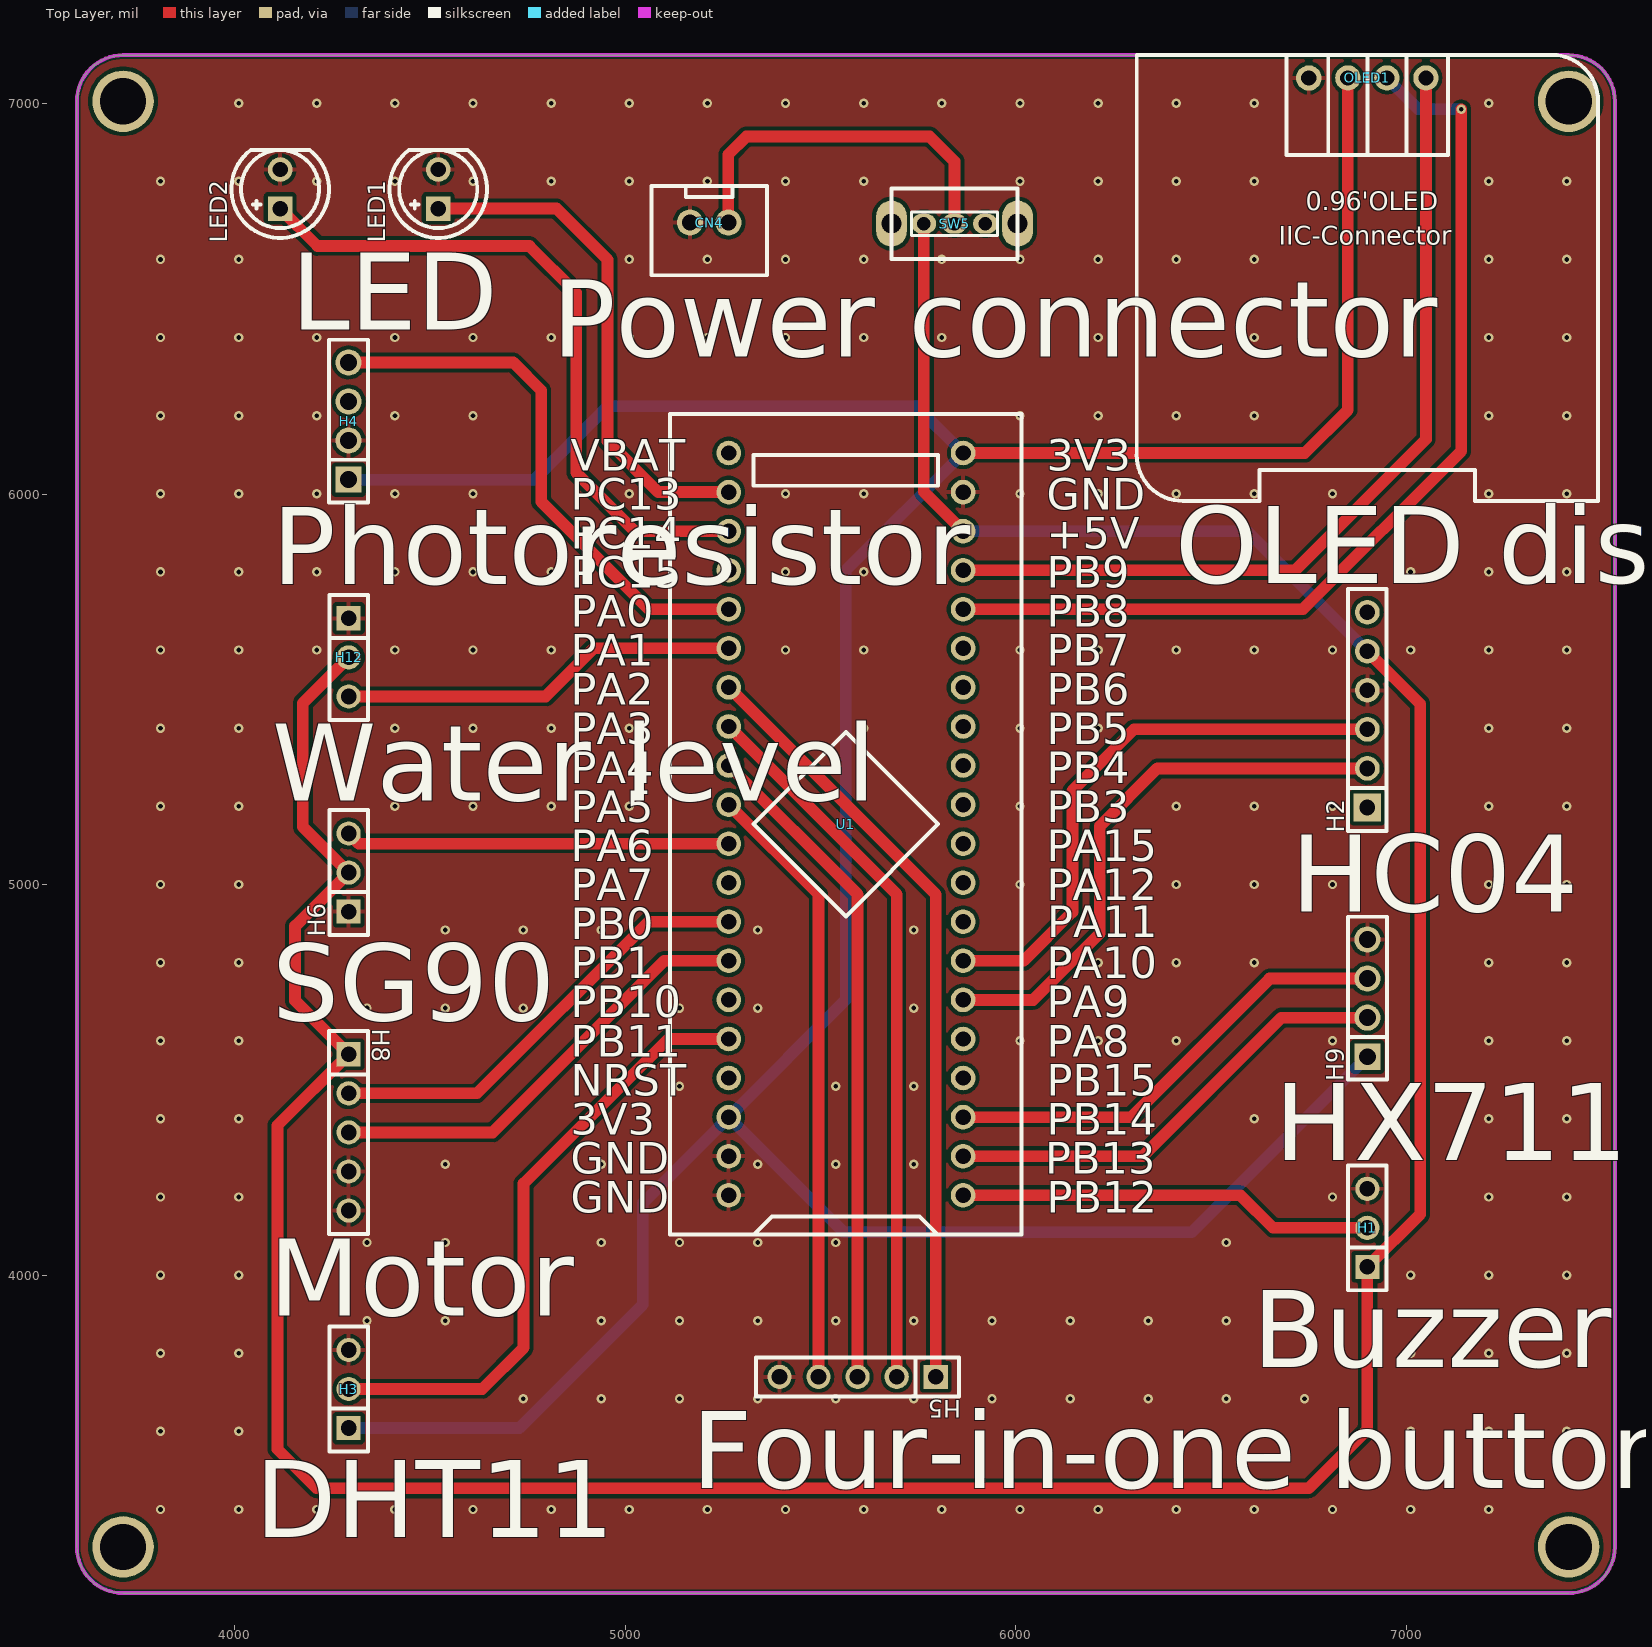
[diagram p0: Top Layer view]
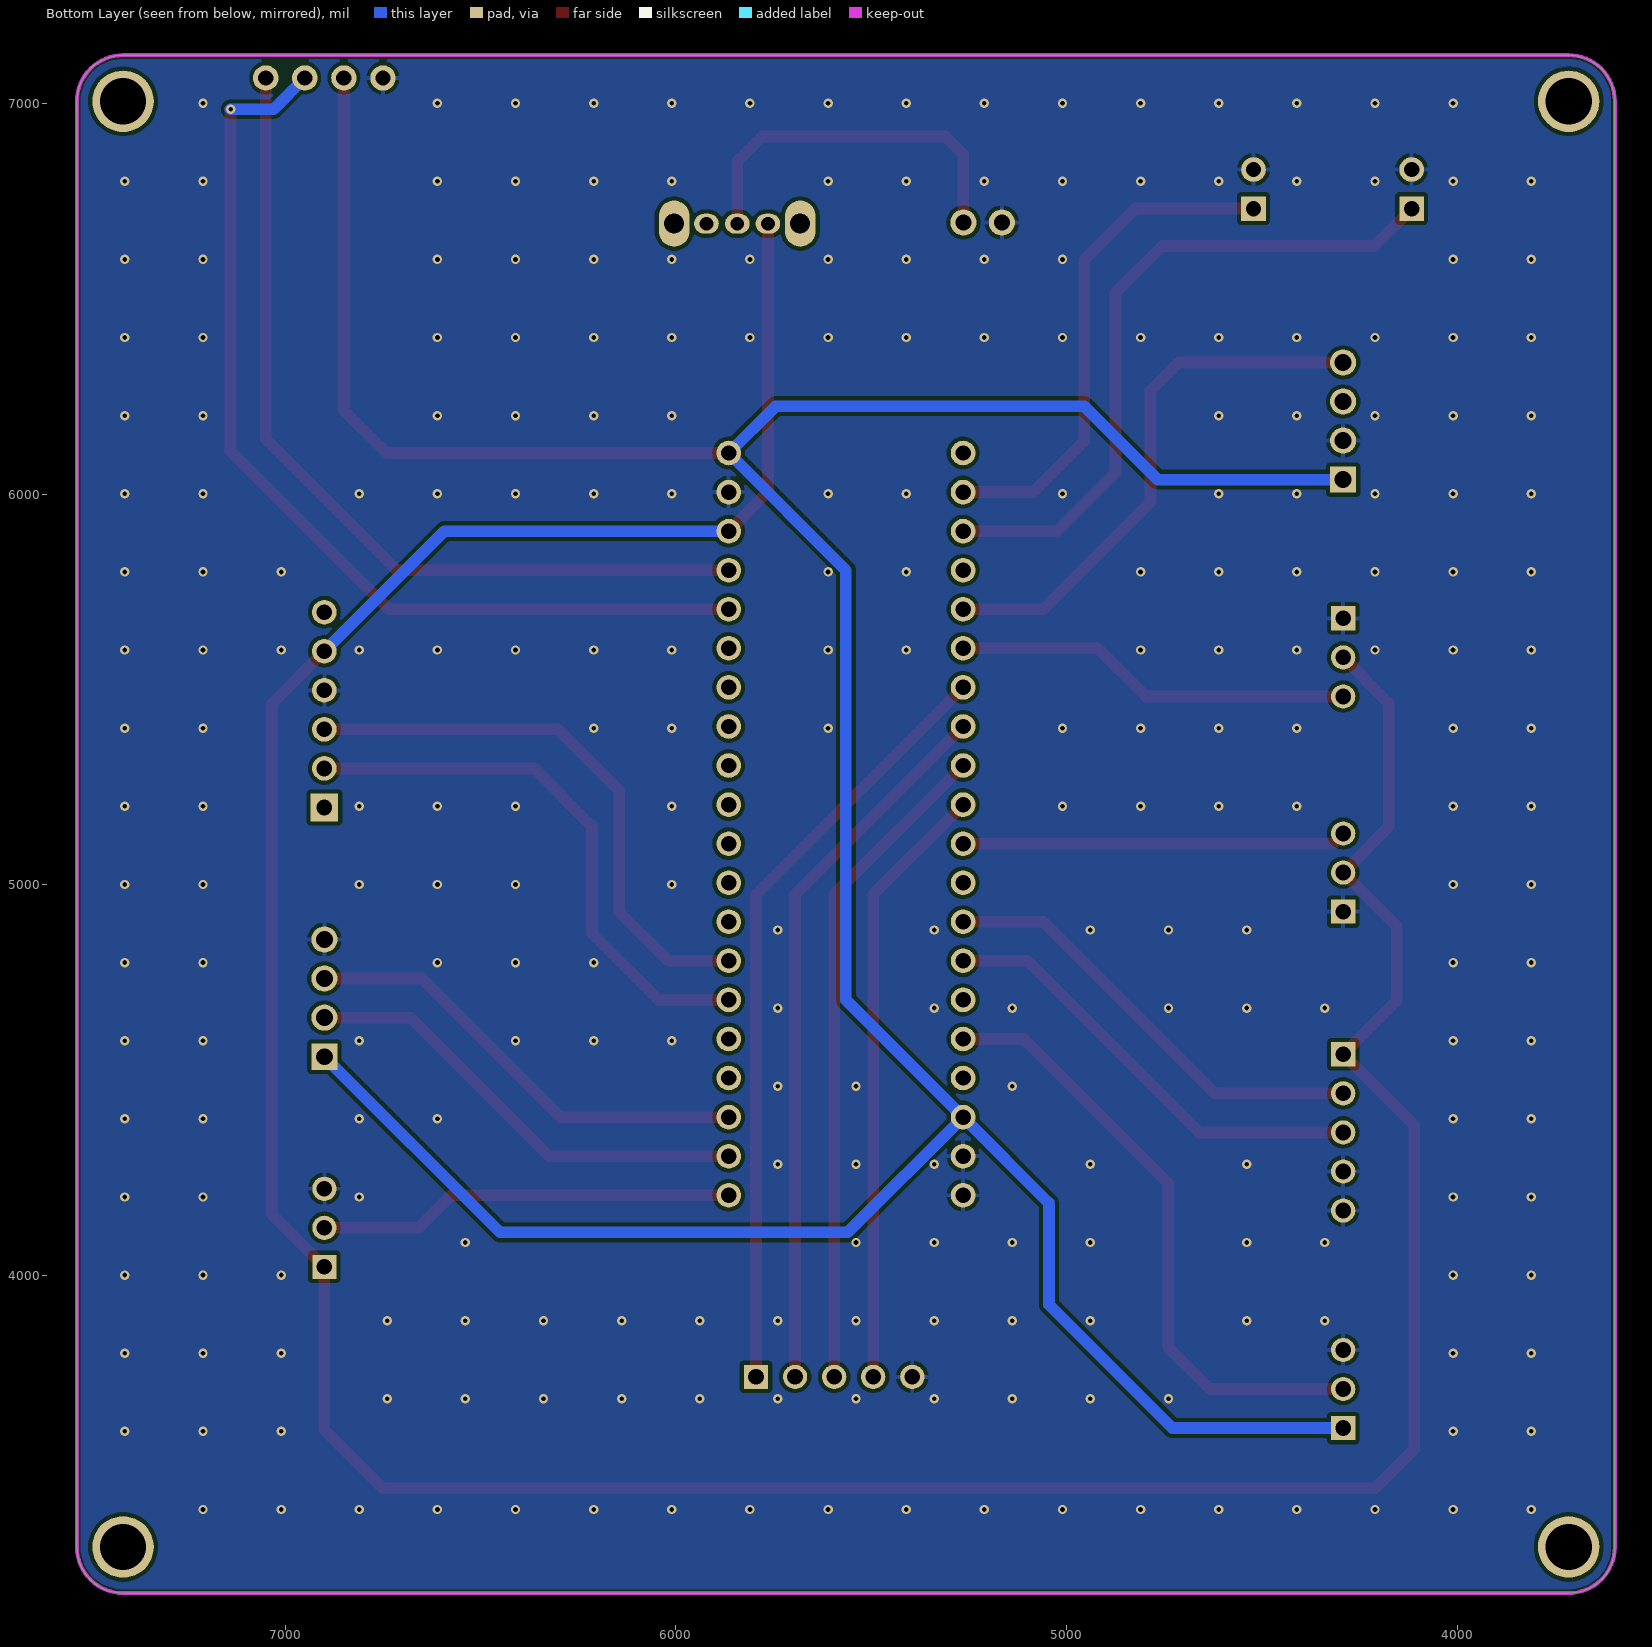
[diagram p1: Bottom Layer view, seen from below]
# Altium PCB MISC51952.pcbdoc
Units mil, origin at the board's own origin, x right, y up, seen from the top; angles counter-clockwise.
Board outline 3937.01 x 3937.01 mil, 2 copper layers (Top Layer, Bottom Layer), stack 62.206 mil thick; 15 components, 38 nets, 95 pads, 254 vias.

## Layer stack, top to bottom
Top Solder Mask Layer: solder mask 0.394, Dk 3.3
Top Layer: signal copper 1.379
Dielectric1: surface 59.449, FR4, Dk 4.5
Bottom Layer: signal copper 1.378
Bottom Solder Mask Layer: solder mask 0.394, Dk 3.3

## Board outline
3714.61,7123.5 ccw(c3714.61,7005.39) 3596.5,7005.39 3596.5,3304.61 ccw(c3714.61,3304.61) 3714.61,3186.5 7415.39,3186.5 ccw(c7415.39,3304.61) 7533.5,3304.61 7533.5,7005.39 ccw(c7415.39,7005.39) 7415.39,7123.5 3714.61,7123.5

## Design rules (kind name [scope] priority, off if disabled: settings)
BoardOutlineClearance copperThickness2oz_1 [All] p2 off: genericclearance=7.99 ignorepadtopadclearanceinfootprint=FALSE except(0: Arc-SplitContinuation Track-SplitContinuation SMDPad-SplitContinuation THPad-SplitContinuation Via-SplitContinuation Fill-SplitContinuation Region-SplitContinuation Poly-SplitContinuation Text-SplitContinuation Hole-SplitContinuation; 5.98: Arc-CutoutEdge Track-CutoutEdge SMDPad-CutoutEdge THPad-CutoutEdge Via-CutoutEdge Text-CutoutEdge; 6.9: Hole-OutlineEdge Hole-CutoutEdge; 10: Poly-OutlineEdge Poly-CutoutEdge; 11.81: Arc-OutlineEdge Track-OutlineEdge SMDPad-OutlineEdge THPad-OutlineEdge Via-OutlineEdge Fill-OutlineEdge Region-OutlineEdge Text-OutlineEdge Fill-CutoutEdge Region-CutoutEdge)
BoardOutlineClearance Plane_innerPlane_1 [All] p4 off: genericclearance=4.02 ignorepadtopadclearanceinfootprint=FALSE except(0: Arc-SplitContinuation Track-SplitContinuation SMDPad-SplitContinuation THPad-SplitContinuation Via-SplitContinuation Fill-SplitContinuation Region-SplitContinuation Poly-SplitContinuation Text-SplitContinuation Hole-SplitContinuation; 5.98: Arc-CutoutEdge Track-CutoutEdge SMDPad-CutoutEdge THPad-CutoutEdge Via-CutoutEdge Text-CutoutEdge; 6.9: Hole-OutlineEdge Hole-CutoutEdge; 10: Poly-OutlineEdge Poly-CutoutEdge; 11.81: Arc-OutlineEdge Track-OutlineEdge SMDPad-OutlineEdge THPad-OutlineEdge Via-OutlineEdge Fill-OutlineEdge Region-OutlineEdge Text-OutlineEdge Fill-CutoutEdge Region-CutoutEdge)
BoardOutlineClearance Copper_copperRegion_1 [All] p6 off: genericclearance=4.02 ignorepadtopadclearanceinfootprint=FALSE except(0: Arc-SplitContinuation Track-SplitContinuation SMDPad-SplitContinuation THPad-SplitContinuation Via-SplitContinuation Fill-SplitContinuation Region-SplitContinuation Poly-SplitContinuation Text-SplitContinuation Hole-SplitContinuation; 5.98: Arc-CutoutEdge Track-CutoutEdge SMDPad-CutoutEdge THPad-CutoutEdge Via-CutoutEdge Text-CutoutEdge; 6.9: Hole-OutlineEdge Hole-CutoutEdge; 10: Poly-OutlineEdge Poly-CutoutEdge; 11.81: Arc-OutlineEdge Track-OutlineEdge SMDPad-OutlineEdge THPad-OutlineEdge Via-OutlineEdge Fill-OutlineEdge Region-OutlineEdge Text-OutlineEdge Fill-CutoutEdge Region-CutoutEdge)
BoardOutlineClearance Copper_copperRegion_copperThickness1oz_1 [All] p8 off: genericclearance=4.02 ignorepadtopadclearanceinfootprint=FALSE except(0: Arc-SplitContinuation Track-SplitContinuation SMDPad-SplitContinuation THPad-SplitContinuation Via-SplitContinuation Fill-SplitContinuation Region-SplitContinuation Poly-SplitContinuation Text-SplitContinuation Hole-SplitContinuation; 5.98: Arc-CutoutEdge Track-CutoutEdge SMDPad-CutoutEdge THPad-CutoutEdge Via-CutoutEdge Text-CutoutEdge; 6.9: Hole-OutlineEdge Hole-CutoutEdge; 10: Poly-OutlineEdge Poly-CutoutEdge; 11.81: Arc-OutlineEdge Track-OutlineEdge SMDPad-OutlineEdge THPad-OutlineEdge Via-OutlineEdge Fill-OutlineEdge Region-OutlineEdge Text-OutlineEdge Fill-CutoutEdge Region-CutoutEdge)
BoardOutlineClearance Copper_copperRegion_Copper_copperRegion_1 [All] p10 off: genericclearance=4.02 ignorepadtopadclearanceinfootprint=FALSE except(0: Arc-SplitContinuation Track-SplitContinuation SMDPad-SplitContinuation THPad-SplitContinuation Via-SplitContinuation Fill-SplitContinuation Region-SplitContinuation Poly-SplitContinuation Text-SplitContinuation Hole-SplitContinuation; 5.98: Arc-CutoutEdge Track-CutoutEdge SMDPad-CutoutEdge THPad-CutoutEdge Via-CutoutEdge Text-CutoutEdge; 6.9: Hole-OutlineEdge Hole-CutoutEdge; 10: Poly-OutlineEdge Poly-CutoutEdge; 11.81: Arc-OutlineEdge Track-OutlineEdge SMDPad-OutlineEdge THPad-OutlineEdge Via-OutlineEdge Fill-OutlineEdge Region-OutlineEdge Text-OutlineEdge Fill-CutoutEdge Region-CutoutEdge)
BoardOutlineClearance copperThickness1oz_1 [All] p12: genericclearance=4.02 ignorepadtopadclearanceinfootprint=FALSE except(0: Arc-SplitContinuation Track-SplitContinuation SMDPad-SplitContinuation THPad-SplitContinuation Via-SplitContinuation Fill-SplitContinuation Region-SplitContinuation Poly-SplitContinuation Text-SplitContinuation Hole-SplitContinuation; 5.98: Arc-CutoutEdge Track-CutoutEdge SMDPad-CutoutEdge THPad-CutoutEdge Via-CutoutEdge Text-CutoutEdge; 6.9: Hole-OutlineEdge Hole-CutoutEdge; 10: Poly-OutlineEdge Poly-CutoutEdge; 11.81: Arc-OutlineEdge Track-OutlineEdge SMDPad-OutlineEdge THPad-OutlineEdge Via-OutlineEdge Fill-OutlineEdge Region-OutlineEdge Text-OutlineEdge Fill-CutoutEdge Region-CutoutEdge)
Clearance copperThickness2oz [All] p1 off: gap=7.99 ignorepadtopadclearanceinfootprint=FALSE except(5.98: SMDPad-Track SMDPad-SMDPad THPad-Track SMDPad-THPad THPad-THPad Track-Via SMDPad-Via THPad-Via Via-Via Fill-SMDPad Region-SMDPad Fill-THPad Region-THPad Fill-Via Region-Via Fill-Fill Fill-Region Region-Region Arc-Track Arc-SMDPad Arc-THPad Arc-Via Fill-Arc Region-Arc Arc-Arc Text-Track SMDPad-Text Text-THPad Text-Via Fill-Text Region-Text Arc-Text Text-Text; 6.9: Hole-Track Hole-SMDPad Hole-THPad Hole-Via Fill-Hole Region-Hole Hole-Arc Hole-Text; 10: Poly-Track Poly-SMDPad Poly-THPad Poly-Via Poly-Fill Poly-Region Poly-Poly Poly-Arc Poly-Text Poly-Hole; 11.81: Fill-Track Region-Track)
Clearance Plane_innerPlane [All] p3 off: gap=4.02 ignorepadtopadclearanceinfootprint=FALSE except(5.98: SMDPad-Track SMDPad-SMDPad THPad-Track SMDPad-THPad THPad-THPad Track-Via SMDPad-Via THPad-Via Via-Via Fill-SMDPad Region-SMDPad Fill-THPad Region-THPad Fill-Via Region-Via Fill-Fill Fill-Region Region-Region Arc-Track Arc-SMDPad Arc-THPad Arc-Via Fill-Arc Region-Arc Arc-Arc Text-Track SMDPad-Text Text-THPad Text-Via Fill-Text Region-Text Arc-Text Text-Text; 6.9: Hole-Track Hole-SMDPad Hole-THPad Hole-Via Fill-Hole Region-Hole Hole-Arc Hole-Text; 10: Poly-Track Poly-SMDPad Poly-THPad Poly-Via Poly-Fill Poly-Region Poly-Poly Poly-Arc Poly-Text Poly-Hole; 11.81: Fill-Track Region-Track)
Clearance Copper_copperRegion [All] p5 off: gap=4.02 ignorepadtopadclearanceinfootprint=FALSE except(5.98: SMDPad-Track SMDPad-SMDPad THPad-Track SMDPad-THPad THPad-THPad Track-Via SMDPad-Via THPad-Via Via-Via Fill-SMDPad Region-SMDPad Fill-THPad Region-THPad Fill-Via Region-Via Fill-Fill Fill-Region Region-Region Arc-Track Arc-SMDPad Arc-THPad Arc-Via Fill-Arc Region-Arc Arc-Arc Text-Track SMDPad-Text Text-THPad Text-Via Fill-Text Region-Text Arc-Text Text-Text; 6.9: Hole-Track Hole-SMDPad Hole-THPad Hole-Via Fill-Hole Region-Hole Hole-Arc Hole-Text; 10: Poly-Track Poly-SMDPad Poly-THPad Poly-Via Poly-Fill Poly-Region Poly-Poly Poly-Arc Poly-Text Poly-Hole; 11.81: Fill-Track Region-Track)
Clearance Copper_copperRegion_copperThickness1oz [All] p7 off: gap=4.02 ignorepadtopadclearanceinfootprint=FALSE except(5.98: SMDPad-Track SMDPad-SMDPad THPad-Track SMDPad-THPad THPad-THPad Track-Via SMDPad-Via THPad-Via Via-Via Fill-SMDPad Region-SMDPad Fill-THPad Region-THPad Fill-Via Region-Via Fill-Fill Fill-Region Region-Region Arc-Track Arc-SMDPad Arc-THPad Arc-Via Fill-Arc Region-Arc Arc-Arc Text-Track SMDPad-Text Text-THPad Text-Via Fill-Text Region-Text Arc-Text Text-Text; 6.9: Hole-Track Hole-SMDPad Hole-THPad Hole-Via Fill-Hole Region-Hole Hole-Arc Hole-Text; 10: Poly-Track Poly-SMDPad Poly-THPad Poly-Via Poly-Fill Poly-Region Poly-Poly Poly-Arc Poly-Text Poly-Hole; 11.81: Fill-Track Region-Track)
Clearance Copper_copperRegion_Copper_copperRegion [All] p9 off: gap=4.02 ignorepadtopadclearanceinfootprint=FALSE except(5.98: SMDPad-Track SMDPad-SMDPad THPad-Track SMDPad-THPad THPad-THPad Track-Via SMDPad-Via THPad-Via Via-Via Fill-SMDPad Region-SMDPad Fill-THPad Region-THPad Fill-Via Region-Via Fill-Fill Fill-Region Region-Region Arc-Track Arc-SMDPad Arc-THPad Arc-Via Fill-Arc Region-Arc Arc-Arc Text-Track SMDPad-Text Text-THPad Text-Via Fill-Text Region-Text Arc-Text Text-Text; 6.9: Hole-Track Hole-SMDPad Hole-THPad Hole-Via Fill-Hole Region-Hole Hole-Arc Hole-Text; 10: Poly-Track Poly-SMDPad Poly-THPad Poly-Via Poly-Fill Poly-Region Poly-Poly Poly-Arc Poly-Text Poly-Hole; 11.81: Fill-Track Region-Track)
Clearance copperThickness1oz [All] p11: gap=4.02 ignorepadtopadclearanceinfootprint=FALSE except(5.98: SMDPad-Track SMDPad-SMDPad THPad-Track SMDPad-THPad THPad-THPad Track-Via SMDPad-Via THPad-Via Via-Via Fill-SMDPad Region-SMDPad Fill-THPad Region-THPad Fill-Via Region-Via Fill-Fill Fill-Region Region-Region Arc-Track Arc-SMDPad Arc-THPad Arc-Via Fill-Arc Region-Arc Arc-Arc Text-Track SMDPad-Text Text-THPad Text-Via Fill-Text Region-Text Arc-Text Text-Text; 6.9: Hole-Track Hole-SMDPad Hole-THPad Hole-Via Fill-Hole Region-Hole Hole-Arc Hole-Text; 10: Poly-Track Poly-SMDPad Poly-THPad Poly-Via Poly-Fill Poly-Region Poly-Poly Poly-Arc Poly-Text Poly-Hole; 11.81: Fill-Track Region-Track)
DiffPairsRouting differentialPair [All] p1: maxlimit=6 minlimit=6 mostfreqgap=6 toplayer_minwidth=5 toplayer_prefwidth=10 toplayer_maxwidth=100 toplayer_mingap=6 toplayer_prefgap=6 toplayer_maxgap=6 bottomlayer_minwidth=5 bottomlayer_prefwidth=10 bottomlayer_maxwidth=100 bottomlayer_mingap=6 bottomlayer_prefgap=6 bottomlayer_maxgap=6 maxuncoupledlength=10
HoleToHoleClearance otherClearance [All] p1: gap=11.81 allowstackedmicrovias=TRUE
Length netLength [All] p1: minlimit=0 maxlimit=0
PasteMaskExpansion pasteMaskExpansion [All] p1: expansion=0
PlaneConnect innerPlane [All] p1: planeconnectstyle=Relief reliefexpansion=20 reliefentries=4 reliefconductorwidth=10 reliefairgap=10
PolygonConnect copperRegion_copperThickness1oz [All] p1 off: connectstyle=Relief reliefconductorwidth=10 reliefentries=4 polygonreliefangle="90 Angle" airgapwidth=10 via.connectstyle=Relief via.reliefconductorwidth=10 via.reliefentries=4 via.polygonreliefangle="90 Angle" via.airgapwidth=10
PolygonConnect copperRegion_Copper_copperRegion [All] p2 off: connectstyle=Relief reliefconductorwidth=10 reliefentries=4 polygonreliefangle="90 Angle" airgapwidth=10 via.connectstyle=Relief via.reliefconductorwidth=10 via.reliefentries=4 via.polygonreliefangle="90 Angle" via.airgapwidth=10
PolygonConnect copperRegion [All] p3: connectstyle=Relief reliefconductorwidth=10 reliefentries=4 polygonreliefangle="90 Angle" airgapwidth=10 via.connectstyle=Relief via.reliefconductorwidth=10 via.reliefentries=4 via.polygonreliefangle="90 Angle" via.airgapwidth=10
RoutingVias viaSize [All] p1: holewidth=12.01 width=24.02 viastyle="Through Hole" minholewidth=11.81 minwidth=19.68 maxholewidth=248.03 maxwidth=393.7
SolderMaskExpansion solderMaskExpansion [IsVia] p1: expansion=-1000 istentingtop=TRUE
SolderMaskExpansion solderMaskExpansion [All] p2: expansion=2 istentingtop=FALSE
Width copperThickness2oz_2 [All] p1 off: maxlimit=100 minlimit=8 preferedwidth=10
Width copperThickness1oz_2 [All] p2: maxlimit=100 minlimit=5 preferedwidth=10

## Components (designator, comment, footprint, x,y, rotation, side; value= is the part's Value field where it differs from the comment)
CN4 "XH2.54*2P_Straight" CONN-TH_2P-P2.50-XH2.54-2P 5215,6695 r0 top
H1 "" HDR-TH_3P-P2.54-V-F 6900,4121.59 r90 top
H2 "" HDR-TH_6P-P2.54-V-F 6900,5447.56 r90 top
H3 "" HDR-TH_3P-P2.54-V-F 4292.04,3708.95 r90 top
H4 "" HDR-TH_4P-P2.54-V-F 4292.04,6186.79 r90 top
H5 "" HDR-TH_5P-P2.54-V-F 5595,3740 r180 top
H6 "" HDR-TH_3P-P2.54-V-F 4292.04,5031.04 r90 top
H8 "" HDR-TH_5P-P2.54-V-F 4292.04,4365.82 r270 top
H9 "" HDR-TH_4P-P2.54-V-F 6900,4709.57 r90 top
H12 "" HDR-TH_3P-P2.54-V-F 4292.04,5581.8 r270 top
LED1 "" LED-TH_5mm 4521.48,6780.67 r90 top
LED2 "" LED-TH_5mm 4116.79,6780.67 r90 top
OLED1 "" 0.96OLED_4P 6900,7065 r0 top
SW5 "" 拨动开关 5837.9,6692.05 r0 top
U1 "STM32F103C8T6-Card" CONN-TH_L53.3-W22.9_STM32F103C8T6-CARD 5565,5155 r90 top

## Footprints (in the part's own frame and the unit in brackets; to place one, negate y for a bottom-side part, rotate by r counter-clockwise, add the part's x,y. Pads: shape width x height; smd on the part's side, far side on the other; paste and mask are expansions set on the pad)
0.96OLED_4P [mm]
  round 1.65 hole 1 copper offset 0,0: 1(-3.81,-0.001) 2(-1.27,0.002) 3(1.27,0.002) 4(3.81,0.002)
  silkscreen extent -15,-27.5 15,1.5
CONN-TH_2P-P2.50-XH2.54-2P [mm]
  round 1.7 hole 1.05 paste+0 mask+0.05: 1(1.25,0) 2(-1.25,0)
  silkscreen extent -3.75,-3.42 3.75,2.37
CONN-TH_L53.3-W22.9_STM32F103C8T6-CARD [mm]
  round 1.6 hole 1: 1(-24.13,-7.62) 2(-21.59,-7.62) 3(-19.05,-7.62) 4(-16.51,-7.62) 5(-13.97,-7.62) 6(-11.43,-7.62) 7(-8.89,-7.62) 8(-6.35,-7.62) 9(-3.81,-7.62) 10(-1.27,-7.62) 11(1.27,-7.62) 12(3.81,-7.62) 13(6.35,-7.62) 14(8.89,-7.62) 15(11.43,-7.62) 16(13.97,-7.62) 17(16.51,-7.62) 18(19.05,-7.62) 19(21.59,-7.62) 20(24.13,-7.62) 21(24.13,7.62) 22(21.59,7.62) 23(19.05,7.62) 24(16.51,7.62) 25(13.97,7.62) 26(11.43,7.62) 27(8.89,7.62) 28(6.35,7.62) 29(3.81,7.62) 30(1.27,7.62) 31(-1.27,7.62) 32(-3.81,7.62) 33(-6.35,7.62) 34(-8.89,7.62) 35(-11.43,7.62) 36(-13.97,7.62) 37(-16.51,7.62) 38(-19.05,7.62) 39(-21.59,7.62) 40(-24.13,7.62)
  silkscreen extent -26.67,-11.43 26.67,11.43
HDR-TH_3P-P2.54-V-F [mil]
  rect 62x62 hole 40.16: 1(-100,0)
  round 62 hole 40.16: 2(0,0) 3(100,0)
  silkscreen extent -160,-49 160,49
HDR-TH_4P-P2.54-V-F [mm]
  rect 1.7x1.7 hole 1.1: 1(-3.81,0)
  round 1.7 hole 1.1: 2(-1.27,0) 3(1.27,0) 4(3.81,0)
  silkscreen extent -5.29,-1.27 5.29,1.27
HDR-TH_5P-P2.54-V-F [mil]
  rect 62x62 hole 40.16: 1(-200,0)
  round 62 hole 40.16: 2(-100,0) 3(0,0) 4(100,0) 5(200,0)
  silkscreen extent -260,-50 260,50
HDR-TH_6P-P2.54-V-F [mm]
  rect 1.8x1.8 hole 1.02: 1(-6.35,0)
  round 1.6 hole 1.02: 2(-3.81,0) 3(-1.27,0) 4(1.27,0) 5(3.81,0) 6(6.35,0)
  silkscreen extent -7.87,-1.25 7.87,1.25
LED-TH_5mm [mm]
  rect 1.6x1.6 hole 1 paste+0 mask+0.051: 1(-1.27,0)
  round 1.6 hole 1 paste+0 mask+0.051: 2(1.27,0)
  silkscreen extent -3.17,-3.17 2.54,3.17
拨动开关 [mil]
  oval 63x51.2 hole 35.4 paste+0 mask+2: 1(-73.4,0) 2(5,0) 3(84,0)
  oval 78.7x118.1 hole 51.2 paste+0 mask+2: 4(166.7,0) 5(-156.1,0)
  silkscreen extent -156,-90 167,90

## Free pads (board coordinates)
  round 157.48 hole 118.11: 1(3714.61,7005.39) 1(3714.61,3304.61) 1(7415.39,7005.39) 1(7415.39,3304.61)

## Via types
v1: diameter 24.02, hole 12, Top Layer to Bottom Layer, 254 vias

## Nets (pads, with @x,y where several pads share a name; then routed paths per layer and width w, separated by ;. In a path a pad name is that pad's centre, name@x,y a point inside that pad or via, vN(x,y) a via of type N, cw(c..) or ccw(c..) an arc to the next point about the centre after c; other vN are vias at no path point)
$1N17118: CN4.1 SW5.2 | length 958
  Top Layer w30: CN4.1 5264.22,6869.22 5310,6915 5780,6915 5842.9,6852.1 SW5.2
+5V: H1.1 H2.5 H6.2 H8.1 H12.2 SW5.1 U1.18 | length 9301.7
  Top Layer w30: H12.2 4175,5464.75 4175,5148.08 H6.2 4155,4894 4155,4702.86 H8.1 4110,4383.78 4110,3555 4210,3455 6750,3455 6900,3605 H1.1 7035,4156.59 7035,5462.56 H2.5 ; SW5.1 5764.5,6005.5 U1.18
  Bottom Layer w30: U1.18 6592.56,5905 H2.5
GND: CN4.2 H1.3 H2.4 H3.3 H4.2 H5.5 H6.1 H8.4 H8.5 H9.4 H12.1 LED1.2 LED2.2 OLED1.1 U1.19 U1.39 U1.40
  other v1: 3810.6,3400.6 4010.6,3400.6 4210.6,3400.6 4410.6,3400.6 4610.6,3400.6 4810.6,3400.6 5010.6,3400.6 5210.6,3400.6 5410.6,3400.6 5610.6,3400.6 5810.6,3400.6 6010.6,3400.6 6210.6,3400.6 6410.6,3400.6 6610.6,3400.6 6810.6,3400.6 7010.6,3400.6 7210.6,3400.6 3810.6,3600.6 4010.6,3600.6 7010.6,3600.6 7210.6,3600.6 7410.6,3600.6 4739.1,3684.1 4939.1,3684.1 5139.1,3684.1 5339.1,3684.1 5539.1,3684.1 5739.1,3684.1 5939.1,3684.1 6139.1,3684.1 6339.1,3684.1 6539.1,3684.1 6739.1,3684.1 3810.6,3800.6 4010.6,3800.6 7010.6,3800.6 7210.6,3800.6 7410.6,3800.6 4339.1,3884.1 4539.1,3884.1 4939.1,3884.1 5139.1,3884.1 5339.1,3884.1 5539.1,3884.1 5739.1,3884.1 5939.1,3884.1 6139.1,3884.1 6339.1,3884.1 6539.1,3884.1 6739.1,3884.1 3810.6,4000.6 4010.6,4000.6 7010.6,4000.6 7210.6,4000.6 7410.6,4000.6 4339.1,4084.1 4539.1,4084.1 4939.1,4084.1 5139.1,4084.1 5339.1,4084.1 5539.1,4084.1 6539.1,4084.1 3810.6,4200.6 4010.6,4200.6 6810.6,4200.6 7210.6,4200.6 7410.6,4200.6 4539.1,4284.1 4939.1,4284.1 5339.1,4284.1 5539.1,4284.1 5739.1,4284.1 3810.6,4400.6 4010.6,4400.6 6610.6,4400.6 6810.6,4400.6 7210.6,4400.6 7410.6,4400.6 5139.1,4484.1 5539.1,4484.1 5739.1,4484.1 3810.6,4600.6 4010.6,4600.6 6010.6,4600.6 6210.6,4600.6 6410.6,4600.6 6810.6,4600.6 7210.6,4600.6 7410.6,4600.6 4339.1,4684.1 4539.1,4684.1 4739.1,4684.1 5139.1,4684.1 5339.1,4684.1 5739.1,4684.1 3810.6,4800.6 4010.6,4800.6 6210.6,4800.6 6410.6,4800.6 6610.6,4800.6 7210.6,4800.6 7410.6,4800.6 4539.1,4884.1 4739.1,4884.1 4939.1,4884.1 5339.1,4884.1 5739.1,4884.1 3810.6,5000.6 4010.6,5000.6 6010.6,5000.6 6410.6,5000.6 6610.6,5000.6 6810.6,5000.6 7210.6,5000.6 7410.6,5000.6 3810.6,5200.6 4010.6,5200.6 4410.6,5200.6 4610.6,5200.6 4810.6,5200.6 5010.6,5200.6 6010.6,5200.6 6410.6,5200.6 6610.6,5200.6 6810.6,5200.6 7210.6,5200.6 7410.6,5200.6 3810.6,5400.6 4010.6,5400.6 4410.6,5400.6 4610.6,5400.6 4810.6,5400.6 5010.6,5400.6 5610.6,5400.6 6010.6,5400.6 6210.6,5400.6 7210.6,5400.6 7410.6,5400.6 3810.6,5600.6 4010.6,5600.6 4210.6,5600.6 4410.6,5600.6 4610.6,5600.6 4810.6,5600.6 5410.6,5600.6 5610.6,5600.6 6010.6,5600.6 6210.6,5600.6 6410.6,5600.6 6610.6,5600.6 6810.6,5600.6 7010.6,5600.6 7210.6,5600.6 7410.6,5600.6 3810.6,5800.6 4010.6,5800.6 4210.6,5800.6 4410.6,5800.6 4610.6,5800.6 4810.6,5800.6 5410.6,5800.6 5610.6,5800.6 7010.6,5800.6 7210.6,5800.6 7410.6,5800.6 3810.6,6000.6 4010.6,6000.6 4210.6,6000.6 4410.6,6000.6 4610.6,6000.6 5010.6,6000.6 5410.6,6000.6 5610.6,6000.6 6010.6,6000.6 6210.6,6000.6 6410.6,6000.6 6610.6,6000.6 6810.6,6000.6 7210.6,6000.6 7410.6,6000.6 3810.6,6200.6 4010.6,6200.6 4210.6,6200.6 4410.6,6200.6 4610.6,6200.6 6010.6,6200.6 6210.6,6200.6 6410.6,6200.6 6610.6,6200.6 7210.6,6200.6 7410.6,6200.6 3810.6,6400.6 4010.6,6400.6 4210.6,6400.6 4410.6,6400.6 4610.6,6400.6 4810.6,6400.6 5010.6,6400.6 5210.6,6400.6 5410.6,6400.6 5610.6,6400.6 5810.6,6400.6 6010.6,6400.6 6210.6,6400.6 6410.6,6400.6 6610.6,6400.6 7210.6,6400.6 7410.6,6400.6 3810.6,6600.6 4010.6,6600.6 5010.6,6600.6 5210.6,6600.6 5410.6,6600.6 5610.6,6600.6 5810.6,6600.6 6010.6,6600.6 6210.6,6600.6 6410.6,6600.6 6610.6,6600.6 7210.6,6600.6 7410.6,6600.6 3810.6,6800.6 4010.6,6800.6 4210.6,6800.6 4410.6,6800.6 4610.6,6800.6 4810.6,6800.6 5010.6,6800.6 5210.6,6800.6 5410.6,6800.6 5610.6,6800.6 6010.6,6800.6 6210.6,6800.6 6410.6,6800.6 6610.6,6800.6 7210.6,6800.6 7410.6,6800.6 4010.6,7000.6 4210.6,7000.6 4410.6,7000.6 4610.6,7000.6 4810.6,7000.6 5010.6,7000.6 5210.6,7000.6 5410.6,7000.6 5610.6,7000.6 5810.6,7000.6 6010.6,7000.6 6210.6,7000.6 6410.6,7000.6 6610.6,7000.6 7210.6,7000.6
NRST: U1.37
PA0: H4.4 U1.25 | length 1401.6
  Top Layer w30: H4.4 4713.21,6336.79 4785,6265 4785,5980 5060,5705 U1.25
PA1: H12.3 U1.26 | length 1024
  Top Layer w30: H12.3 4796.8,5481.8 4920,5605 U1.26
PA2: H5.1 U1.27 | length 1984.5
  Top Layer w30: U1.27 5795,4975 H5.1
PA3: H5.2 U1.28 | length 1843.1
  Top Layer w30: U1.28 5695,4975 H5.2
PA4: H5.3 U1.29 | length 1701.7
  Top Layer w30: U1.29 5595,4975 H5.3
PA5: H5.4 U1.30 | length 1560.3
  Top Layer w30: U1.30 5495,4975 H5.4
PA6: H6.3 U1.31 | length 983.7
  Top Layer w30: H6.3 4318.08,5105 U1.31
PA7: U1.32
PA8: U1.5
PA9: H2.2 U1.6 | length 1441.5
  Top Layer w30: U1.6 6045,4705 6215,4875 6215,5150 6362.56,5297.56 H2.2
PA10: H2.3 U1.7 | length 1462
  Top Layer w30: U1.7 6020,4805 6145,4930 6145,5240 6302.56,5397.56 H2.3
PA11: U1.8
PA12: U1.9
PA15: U1.10
PB0: H8.2 U1.33 | length 1154.9
  Top Layer w30: H8.2 4620.82,4465.82 5060,4905 U1.33
PB1: H8.3 U1.34 | length 1154.9
  Top Layer w30: H8.3 4660.82,4365.82 5100,4805 U1.34
PB3: U1.11
PB4: U1.12
PB5: U1.13
PB6: U1.14
PB7: U1.15
PB8: OLED1.3 U1.16 | length 2540.9
  Top Layer w30: U1.16 6735,5705 7140,6110 v1(7140,6985)
  Bottom Layer w30: OLED1.3@6950,7065.05 7030.05,6985 v1(7140,6985)
PB9: OLED1.4 U1.17 | length 2248.8
  Top Layer w30: U1.17 6715,5805 7050,6140 OLED1.4@7050,7065.05
PB10: U1.35
PB11: H3.2 U1.36 | length 1590.1
  Top Layer w30: H3.2 4633.95,3708.95 4740,3815 4740,4235 5110,4605 U1.36
PB12: H1.2 U1.1 | length 1069.5
  Top Layer w30: U1.1 6575,4205 6658.41,4121.59 H1.2
PB13: H9.2 U1.2 | length 1181.9
  Top Layer w30: U1.2 6325,4305 6679.57,4659.57 H9.2
PB14: H9.3 U1.3 | length 1181.9
  Top Layer w30: U1.3 6295,4405 6649.57,4759.57 H9.3
PB15: U1.4
PC13: LED1.1 U1.22 | length 1316.5
  Top Layer w30: LED1.1 4824.33,6730.67 4955,6600 4955,6135 5085,6005 U1.22
PC14: LED2.1 U1.23 | length 1759.7
  Top Layer w30: LED2.1 4212.46,6635 4755,6635 4875,6515 4875,6055 5025,5905 U1.23
PC15: U1.24
VBAT: U1.21
VCC: H3.1 H4.1 H9.1 OLED1.2 U1.20 U1.38 | length 8928.2
  Top Layer w30: U1.20 6740,6105 6850,6215 OLED1.2@6850,7065.05
  Bottom Layer w30: H3.1 4728.95,3608.95 5045,3925 5045,4185 U1.38 ; H4.1 4766.79,6036.79 4955,6225 5745,6225 U1.20 5565,5805 5565,4705 U1.38 ; H9.1 6450.42,4110 5560,4110 U1.38
pads on no net: H2.1 H2.6 H4.3 SW5.3 SW5.4 SW5.5

## Polygon pours and split planes (outlines as drawn)
GND on Bottom Layer (solid, remove dead copper, pour order 2): 3525,7245 3525,3080 7700,3080 7700,7245
GND on Top Layer (solid, remove dead copper, pour order 2): 3000,7415 3000,3000 7930,3000 7930,7415

## Keep-outs
Board Outline Layer:
  the board outline again, w10

## Silkscreen, mask and mechanical layers (free items; w line width, h text height)
Top Silkscreen Layer:
  text "LED" at 4145,6420 h196.85
  text "Power connector" at 4812.87,6351.57 h196.85
  text "VBAT" at 4860.95,6060 h80
  text "3V3" at 6079.16,6060 h80
  text "PC13" at 4860.95,5960 h80
  text "GND" at 6079.16,5960 h80
  text "PC14" at 4860.95,5860 h80
  text "+5V" at 6079.16,5860 h80
  text "OLED display" at 6408.02,5771.45 h196.85
  text "Photoresistor" at 4096.23,5769.56 h196.85
  text "PC15" at 4860.95,5760 h80
  text "PB9" at 6079.16,5760 h80
  text "PA0" at 4860.95,5660 h80
  text "PB8" at 6079.16,5660 h80
  text "PA1" at 4860.95,5560 h80
  text "PB7" at 6079.16,5560 h80
  text "PA2" at 4860.95,5460 h80
  text "PB6" at 6079.16,5460 h80
  text "PA3" at 4860.95,5360 h80
  text "PB5" at 6079.16,5360 h80
  text "PA4" at 4860.95,5260 h80
  text "PB4" at 6079.16,5260 h80
  text "Water level" at 4096.68,5214.93 h196.85
  text "PA5" at 4860.95,5160 h80
  text "PB3" at 6079.16,5160 h80
  text "PA6" at 4860.95,5060 h80
  text "PA15" at 6079.16,5060 h80
  text "PA7" at 4860.95,4960 h80
  text "PA12" at 6079.16,4960 h80
  text "HC04" at 6705.38,4931.3 h196.85
  text "PA11" at 6080.95,4865 h80
  text "PB0" at 4860.95,4860 h80
  text "PB1" at 4860.95,4760 h80
  text "PA10" at 6079.16,4760 h80
  text "PB10" at 4860.95,4660 h80
  text "PA9" at 6079.16,4660 h80
  text "SG90" at 4096.09,4651.79 h196.85
  text "PB11" at 4860.95,4560 h80
  text "PA8" at 6079.16,4560 h80
  text "NRST" at 4860.95,4460 h80
  text "PB15" at 6079.16,4460 h80
  text "3V3" at 4860.95,4360 h80
  text "PB14" at 6079.16,4360 h80
  text "HX711" at 6662.43,4294.88 h196.85
  text "GND" at 4860.95,4260 h80
  text "PB13" at 6075.95,4260 h80
  text "GND" at 4860.95,4160 h80
  text "PB12" at 6079.16,4160 h80
  text "Motor" at 4088.93,3896.41 h196.85
  text "Buzzer" at 6606.81,3764.56 h196.85
  text "Four-in-one button" at 5170,3455 h196.85
  text "DHT11" at 4053.43,3330 h196.85